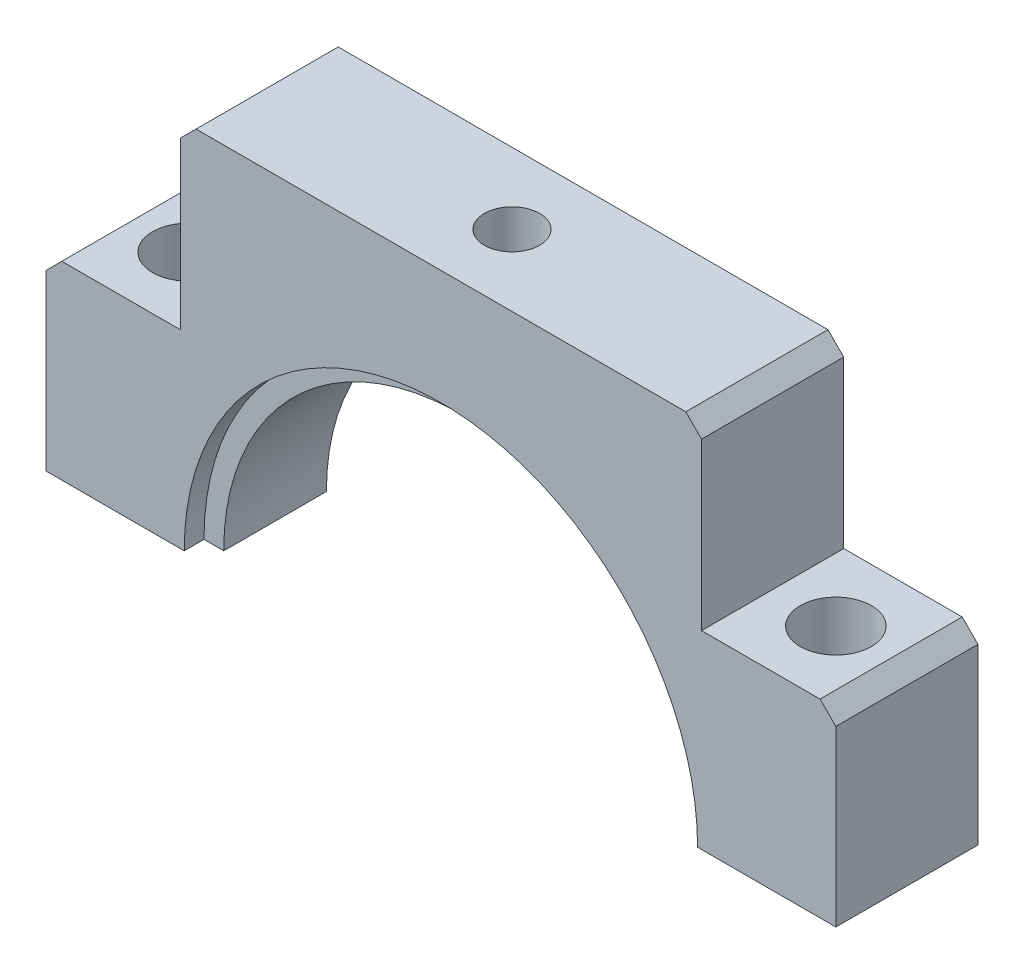
SolidWorks part; units mm, degrees
material "Q235-A"
ref_plane "Front Plane" through (0, 0, 0) normal (0, 0, 1) x (1, 0, 0)
ref_plane "Top Plane" through (0, 0, 0) normal (0, 1, 0) x (1, 0, 0)
ref_plane "Right Plane" through (0, 0, 0) normal (1, 0, 0) x (0, 0, -1)
sketch "Sketch1" plane through (0, 0, 0) normal (0, 0, 1) x (1, 0, 0)
  line L0 (-50, 24) -> (-33, 24)
  line L1 (-50, 0) -> (-30, 0)
  line L2 (-50, 0) -> (-50, 24)
  line L3 (-33, 47) -> (33, 47)
  line L5 (-33, 24) -> (-33, 47)
  line L6 (0, 58.7143) -> (0, -17.0907) construction
  line L7 (50, 0) -> (50, 24)
  line L8 (50, 24) -> (33, 24)
  line L9 (33, 24) -> (33, 47)
  line L10 (30, 0) -> (50, 0)
  arc A0 (30, 0) -> (-30, 0) centre (0, 0) ccw
  point P13 (0, 47)
  dimension "D1" = 100
  dimension "D2" = 47
  dimension "D3" = 23
  dimension "D4" = 33
extrude "Boss-Extrude1" add sketch "Sketch1" along normal blind 18
chamfer "Chamfer1" distance 2 angle 45 4 edges at (50, 24, 9) (33, 47, 9) (-33, 47, 9) (-50, 24, 9)
sketch "Sketch2" plane through (0, 47, 0) normal (0, 1, 0) x (1, 0, 0)
  line L0 (50, -9) -> (-50, -9)
  line L2 (50, 0) -> (50, -18) construction
  line L3 (-50, -18) -> (-50, 0) construction
  line L4 (-41, 0.9192) -> (-41, -18.9192)
  line L5 (41, 0.9192) -> (41, -18.9192)
  point P10 (-41, -9)
  point P11 (41, -9)
  dimension "D1" = 100
  dimension "D2" = 82
  dimension "D3" = 9
hole_wizard "M8x1.0 Tapped Hole1" positions "Sketch3" profile "Sketch4" tap size "M8x1.0" standard "GB"
sketch "Sketch3" plane through (0, 47, 0) normal (0, 1, 0) x (1, 0, 0)
  line L0 (50, -9) -> (-50, -9) construction
  point P0 (0, -9)
sketch "Sketch4" plane through (0, 47, 9) normal (1, 0, 0) x (0, 0, 1)
  line L0 (0, 0) -> (0, 15.103)
  line L1 (0, 15.103) -> (3.5, 13)
  line L2 (3.5, 13) -> (3.5, 0)
  line L5 (3.5, 0) -> (0, 0)
  line L10 (0, 15.103) -> (-3.5, 13) construction
  line L11 (0, -6.35) -> (0, 107.95) construction
  dimension "螺纹孔钻头直径" = 7
  dimension "螺纹孔钻头深度" = 13
  dimension "导头角度" = 118
cosmetic thread "Cosmetic Thread1" parameters "D1"=8, "D2"=8
hole_wizard "Hole2" positions "Sketch9" profile "Sketch10" legacy end condition through all
sketch "Sketch9" plane through (0, 24, 0) normal (0, 1, 0) x (1, 0, 0)
  line L0 (-41, 0.9192) -> (-41, -18.9192) construction
  line L1 (41, 0.9192) -> (41, -18.9192) construction
  point P0 (-41, -9)
  point P4 (41, -9)
sketch "Sketch10" plane through (-41, 24, 9) normal (1, 0, 0) x (0, 0, 1)
  line L0 (0, 0) -> (0, 24)
  line L1 (0, 24) -> (4.5, 24)
  line L2 (4.5, 24) -> (4.5, 0)
  line L3 (4.5, 0) -> (0, 0)
  line L4 (0, 110) -> (0, -10) construction
  dimension "直径" = 9
  dimension "深度" = 24
sketch "Sketch15" plane through (0, 0, 0) normal (0, 0, -1) x (-1, 0, 0)
  circle A0 centre (0, 0) radius 32.5
extrude "Cut-Extrude3" cut sketch "Sketch15" against normal blind 2.5
sketch "Sketch16" plane through (0, 0, 18) normal (0, 0, 1) x (1, 0, 0)
  circle A1 centre (0, 0) radius 32.5
  circle A2 centre (0, 0) radius 32.5
  dimension "D1" = 0
extrude "Cut-Extrude4" cut sketch "Sketch16" against normal blind 2.5
hole_wizard "Hole3" positions "Sketch17" profile "Sketch18" legacy end condition through all
sketch "Sketch17" plane through (0, 47, 0) normal (0, 1, 0) x (1, 0, 0)
  point P0 (0, -9)
sketch "Sketch18" plane through (0, 47, 9) normal (1, 0, 0) x (0, 0, 1)
  line L0 (0, 0) -> (0, 47)
  line L1 (0, 47) -> (2, 47)
  line L2 (2, 47) -> (2, 0)
  line L3 (2, 0) -> (0, 0)
  line L4 (0, 110) -> (0, -10) construction
  dimension "直径" = 4
  dimension "深度" = 47
